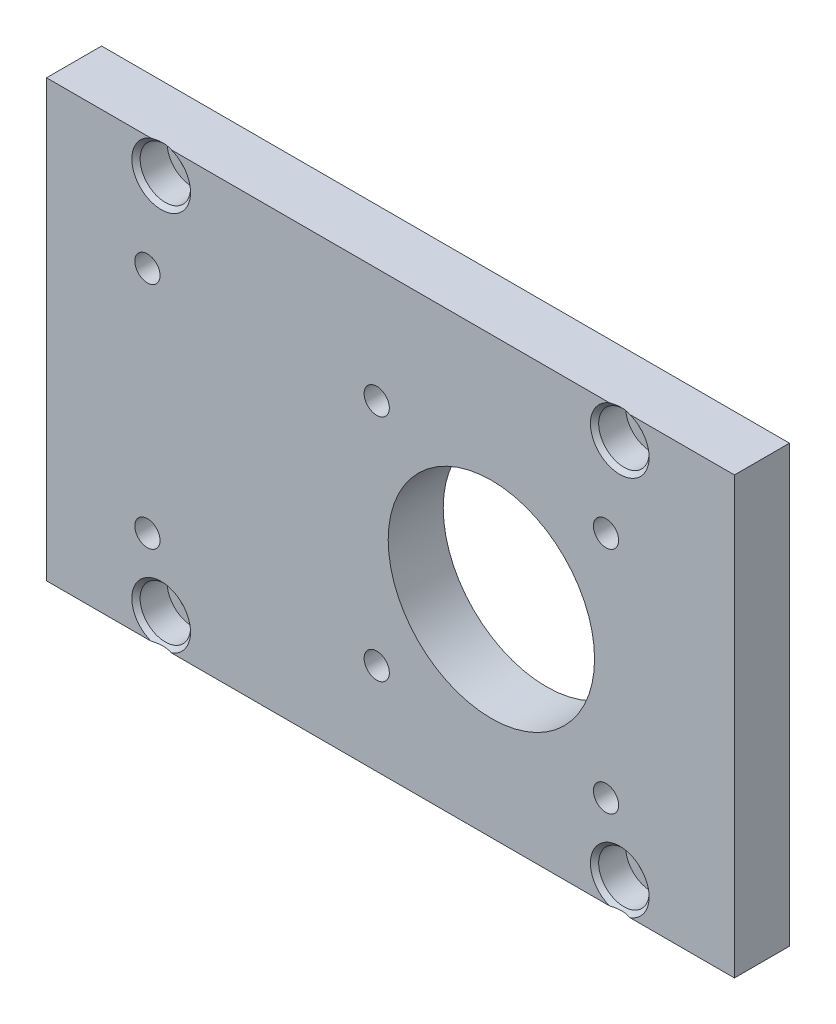
SolidWorks part; units mm, degrees
material "6061 合金"
ref_plane "前视基准面" through (0, 0, 0) normal (0, 0, 1) x (1, 0, 0)
ref_plane "上视基准面" through (0, 0, 0) normal (0, 1, 0) x (1, 0, 0)
ref_plane "右视基准面" through (0, 0, 0) normal (1, 0, 0) x (0, 0, -1)
sketch "草图1" plane through (0, 0, 0) normal (0, 0, 1) x (1, 0, 0)
  line L1 (-75, 47.5) -> (75, 47.5)
  line L2 (-75, 47.5) -> (-75, -47.5)
  line L3 (-75, -47.5) -> (75, -47.5)
  line L4 (75, 47.5) -> (75, -47.5)
  line L5 (-75, 47.5) -> (75, -47.5) construction
  line L6 (-75, -47.5) -> (75, 47.5) construction
  point P0 (0, 0)
  dimension "D1" = 150
  dimension "D2" = 95
extrude "凸台-拉伸1" add sketch "草图1" along normal blind 12
hole_wizard "打孔尺寸(%根据)内六角圆柱头螺钉的类型1" positions "草图4" profile "草图6" counterbore size "M6" standard "GB" end condition through all
sketch "草图4" plane through (0, 0, 12) normal (0, 0, 1) x (1, 0, 0)
  point P3 (-50, -41.5)
  point P6 (50, -41.5)
  point P9 (-50, 41.5)
  point P12 (50, 41.5)
sketch "草图6" plane through (-50, -41.5, 12) normal (1, 0, 0) x (0, -1, 0)
  line L0 (0, 0) -> (0, 12)
  line L1 (0, 12) -> (3.3, 12)
  line L3 (3.3, 12) -> (3.3, 6.8)
  line L4 (5.5, 6.8) -> (3.3, 6.8)
  line L5 (5.5, 6.8) -> (5.5, 0.9)
  line L6 (5.5, 0.9) -> (6.4, 0)
  line L7 (6.4, 0) -> (0, 0)
  line L8 (-5.5, 0.9) -> (-6.4, 0) construction
  line L11 (0, -6.35) -> (0, 107.95) construction
  dimension "通孔孔直径" = 6.6
  dimension "通孔孔深度" = 12
  dimension "柱形沉头孔直径" = 11
  dimension "柱形沉头孔深度" = 6.8
  dimension "近端锥形沉头孔直径" = 12.8
  dimension "近端锥形沉头孔角度" = 90
hole_wizard "打孔尺寸(%根据)内六角圆柱头螺钉的类型2" positions "草图7" profile "草图8" counterbore size "M5" standard "GB" end condition through all
sketch "草图7" plane through (0, 0, 0) normal (0, 0, -1) x (-1, 0, 0)
  point P2 (53, -27.5)
  point P5 (3, -27.5)
  point P8 (-47, -27.5)
  point P11 (-47, 22.5)
  point P14 (3, 22.5)
  point P17 (53, 22.5)
sketch "草图8" plane through (-53, -27.5, 0) normal (1, 0, 0) x (0, 1, 0)
  line L0 (0, 0) -> (0, 12)
  line L1 (0, 12) -> (2.75, 12)
  line L3 (2.75, 12) -> (2.75, 5.7)
  line L4 (5, 5.7) -> (2.75, 5.7)
  line L5 (5, 5.7) -> (5, 0.025)
  line L6 (5, 0.025) -> (5.025, 0)
  line L7 (5.025, 0) -> (0, 0)
  line L8 (-5, 0.025) -> (-5.025, 0) construction
  line L11 (0, -6.35) -> (0, 107.95) construction
  dimension "通孔孔直径" = 5.5
  dimension "通孔孔深度" = 12
  dimension "柱形沉头孔直径" = 10
  dimension "柱形沉头孔深度" = 5.7
  dimension "近端锥形沉头孔直径" = 10.05
  dimension "近端锥形沉头孔角度" = 90
sketch "草图9" plane through (0, 0, 0) normal (0, 0, -1) x (-1, 0, 0)
  circle A0 centre (-22, -2.5) radius 22.5
  dimension "D1" = 45
extrude "切除-拉伸1" cut sketch "草图9" against normal through all
